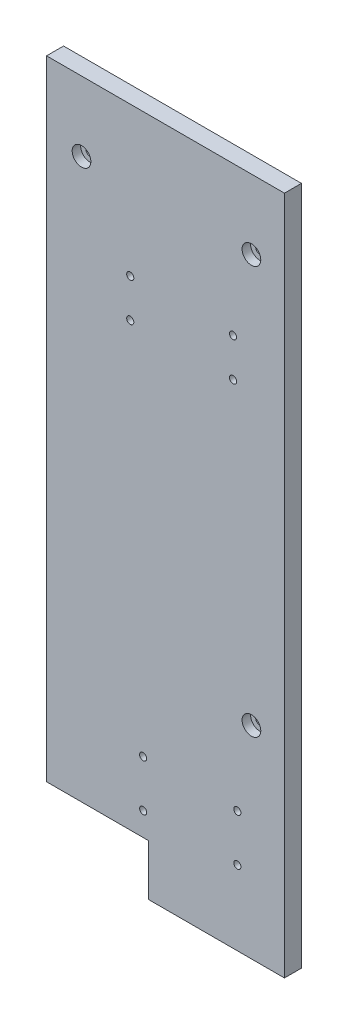
from build123d import *

# Parameters (mm, degrees)
EXTRUDE_1_DEPTH     = 10
SKETCH_10_R         = 2.5
SKETCH_10_R_2       = 2.1
CUT_EXTRUDE_1_DEPTH = 10
SKETCH_11_R         = 5.5
CUT_EXTRUDE_2_DEPTH = 5


with BuildPart() as part:
    # 草图1 → 凸台-拉伸1 (new body)
    with BuildSketch(Plane.XY):
        Polygon((-99.58041958, -70.769230769), (-39.58041958, -70.769230769), (-39.58041958, -100.769230769), (40.41958042, -100.769230769), (40.41958042, 299.230769231), (-99.58041958, 299.230769231), align=None)
    extrude(amount=EXTRUDE_1_DEPTH)

    # 草图10 → 切除-拉伸1 (cut)
    with BuildSketch(Plane.XY.offset(10)):
        with Locations((-79.008794304, 258.253022412)):
            Circle(SKETCH_10_R)
        with Locations((20.991205696, 258.253022412)):
            Circle(SKETCH_10_R)
        with Locations((-50.330419577, 211.582541175)):
            Circle(SKETCH_10_R_2)
        with Locations((-50.330419577, 189.082541175)):
            Circle(SKETCH_10_R_2)
        with Locations((10.169580423, 211.582541175)):
            Circle(SKETCH_10_R_2)
        with Locations((10.169580423, 189.082541175)):
            Circle(SKETCH_10_R_2)
        with Locations((-42.717061736, -29.519230769)):
            Circle(SKETCH_10_R_2)
        with Locations((-42.717061736, -57.019230769)):
            Circle(SKETCH_10_R_2)
        with Locations((12.707366369, -57.019230769)):
            Circle(SKETCH_10_R_2)
        with Locations((12.707366369, -29.519230769)):
            Circle(SKETCH_10_R_2)
        with Locations((20.991205696, 18.253022412)):
            Circle(SKETCH_10_R)
    extrude(amount=-CUT_EXTRUDE_1_DEPTH, mode=Mode.SUBTRACT)

    # 草图11 → 切除-拉伸2 (cut)
    with BuildSketch(Plane(origin=(-949.724352481, 990.975018952, 10), x_dir=(0, -1, 0), z_dir=(0, 0, 1))):
        with Locations(Location((732.680785462, 870.715566681, 0), (0, 0, 90))):
            Circle(SKETCH_11_R)
        with Locations(Location((732.72199654, 970.71555819, 0), (0, 0, 90))):
            Circle(SKETCH_11_R)
        with Locations(Location((972.72199654, 970.71555819, 0), (0, 0, 90))):
            Circle(SKETCH_11_R)
    extrude(amount=-CUT_EXTRUDE_2_DEPTH, mode=Mode.SUBTRACT)


solid = part.part
